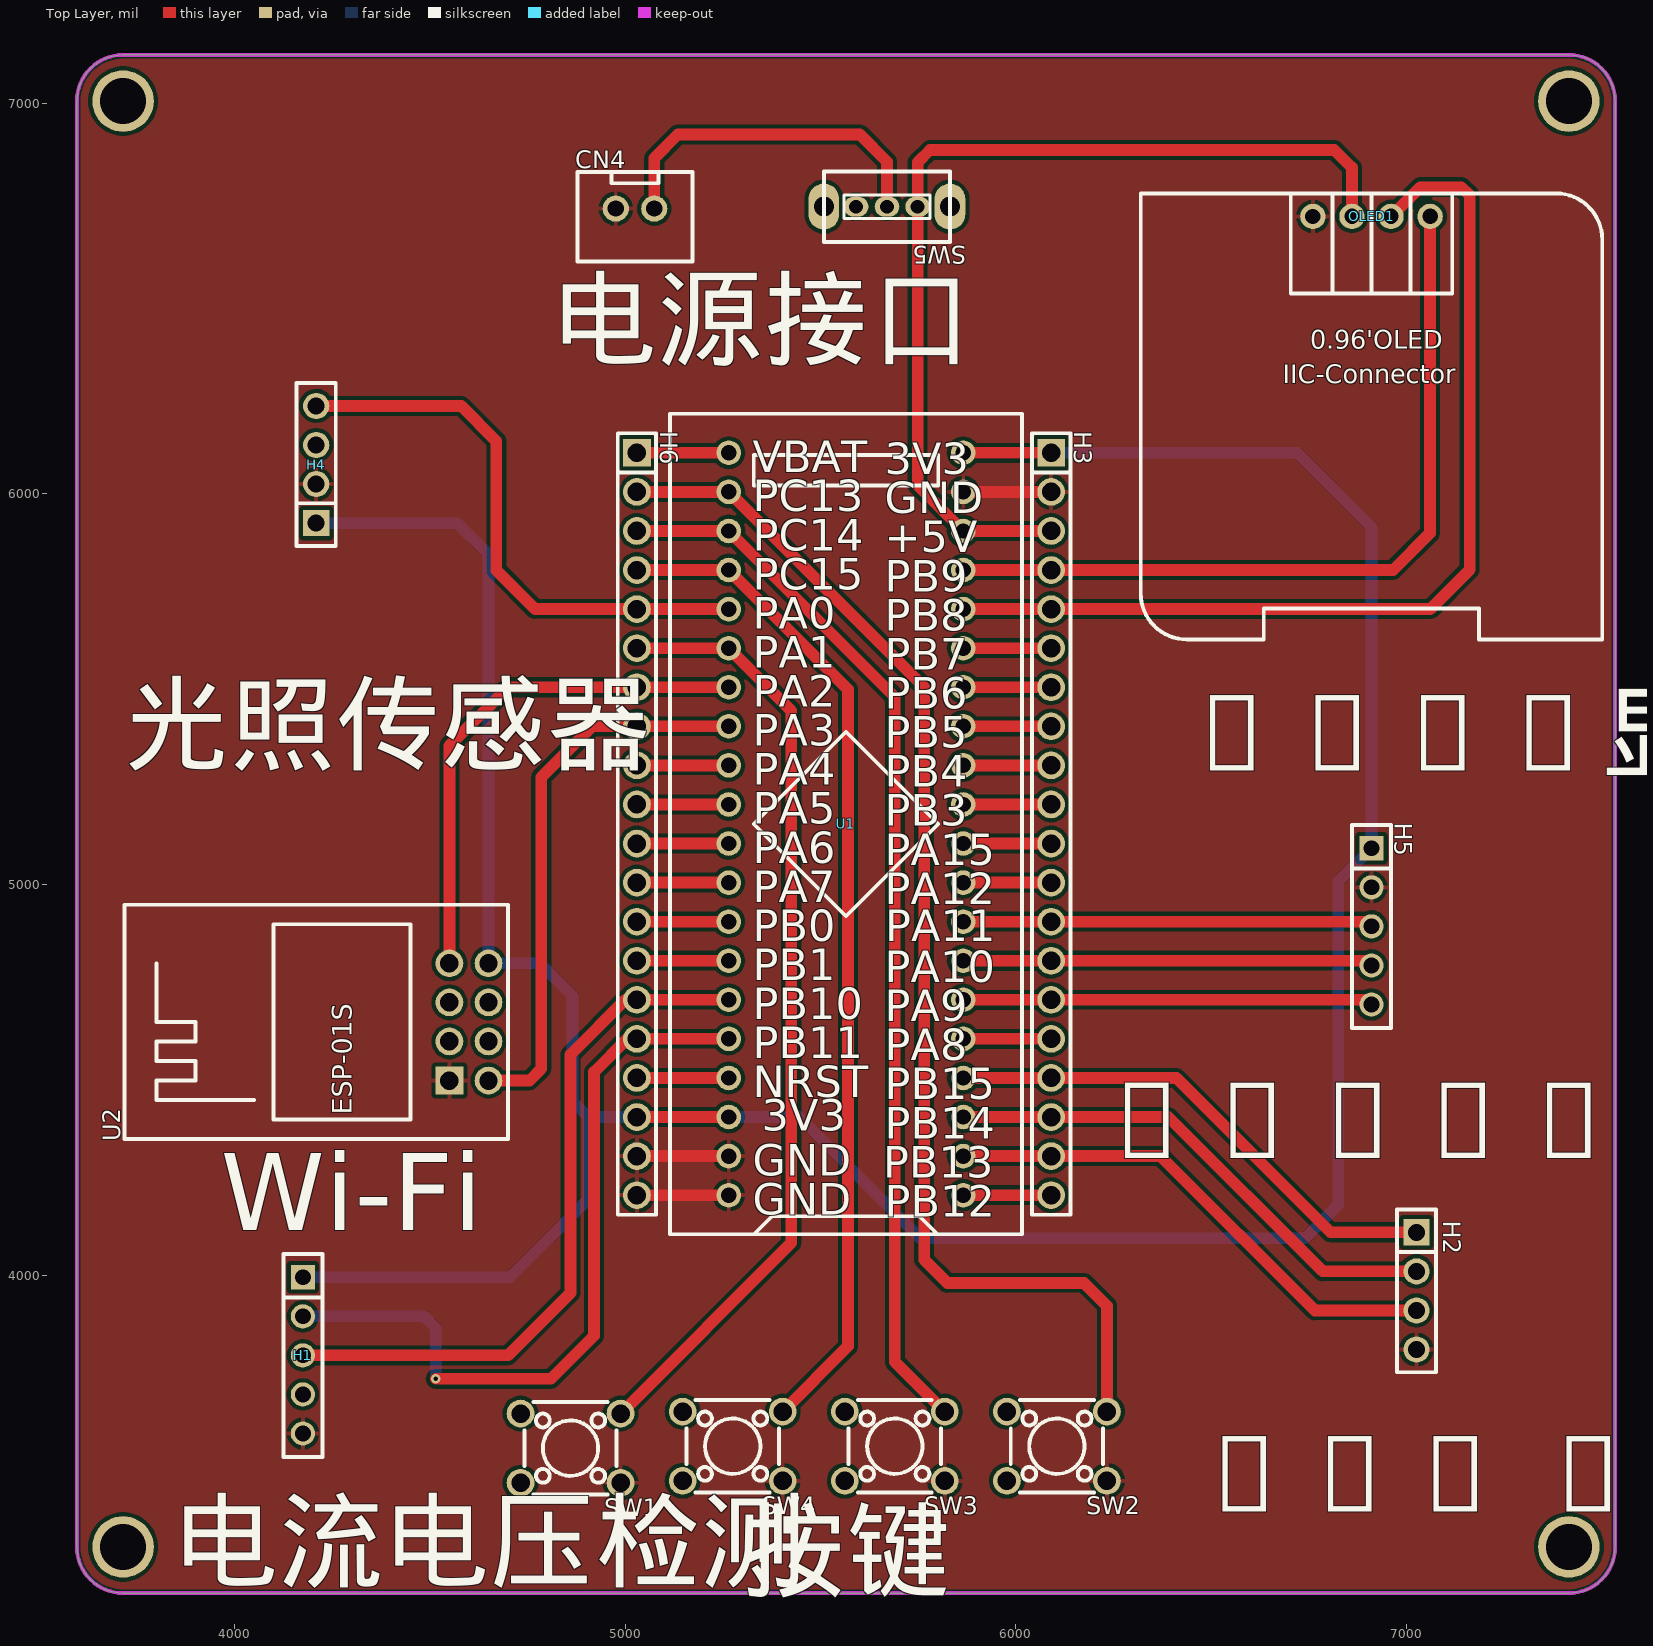
[diagram p0: Top Layer view]
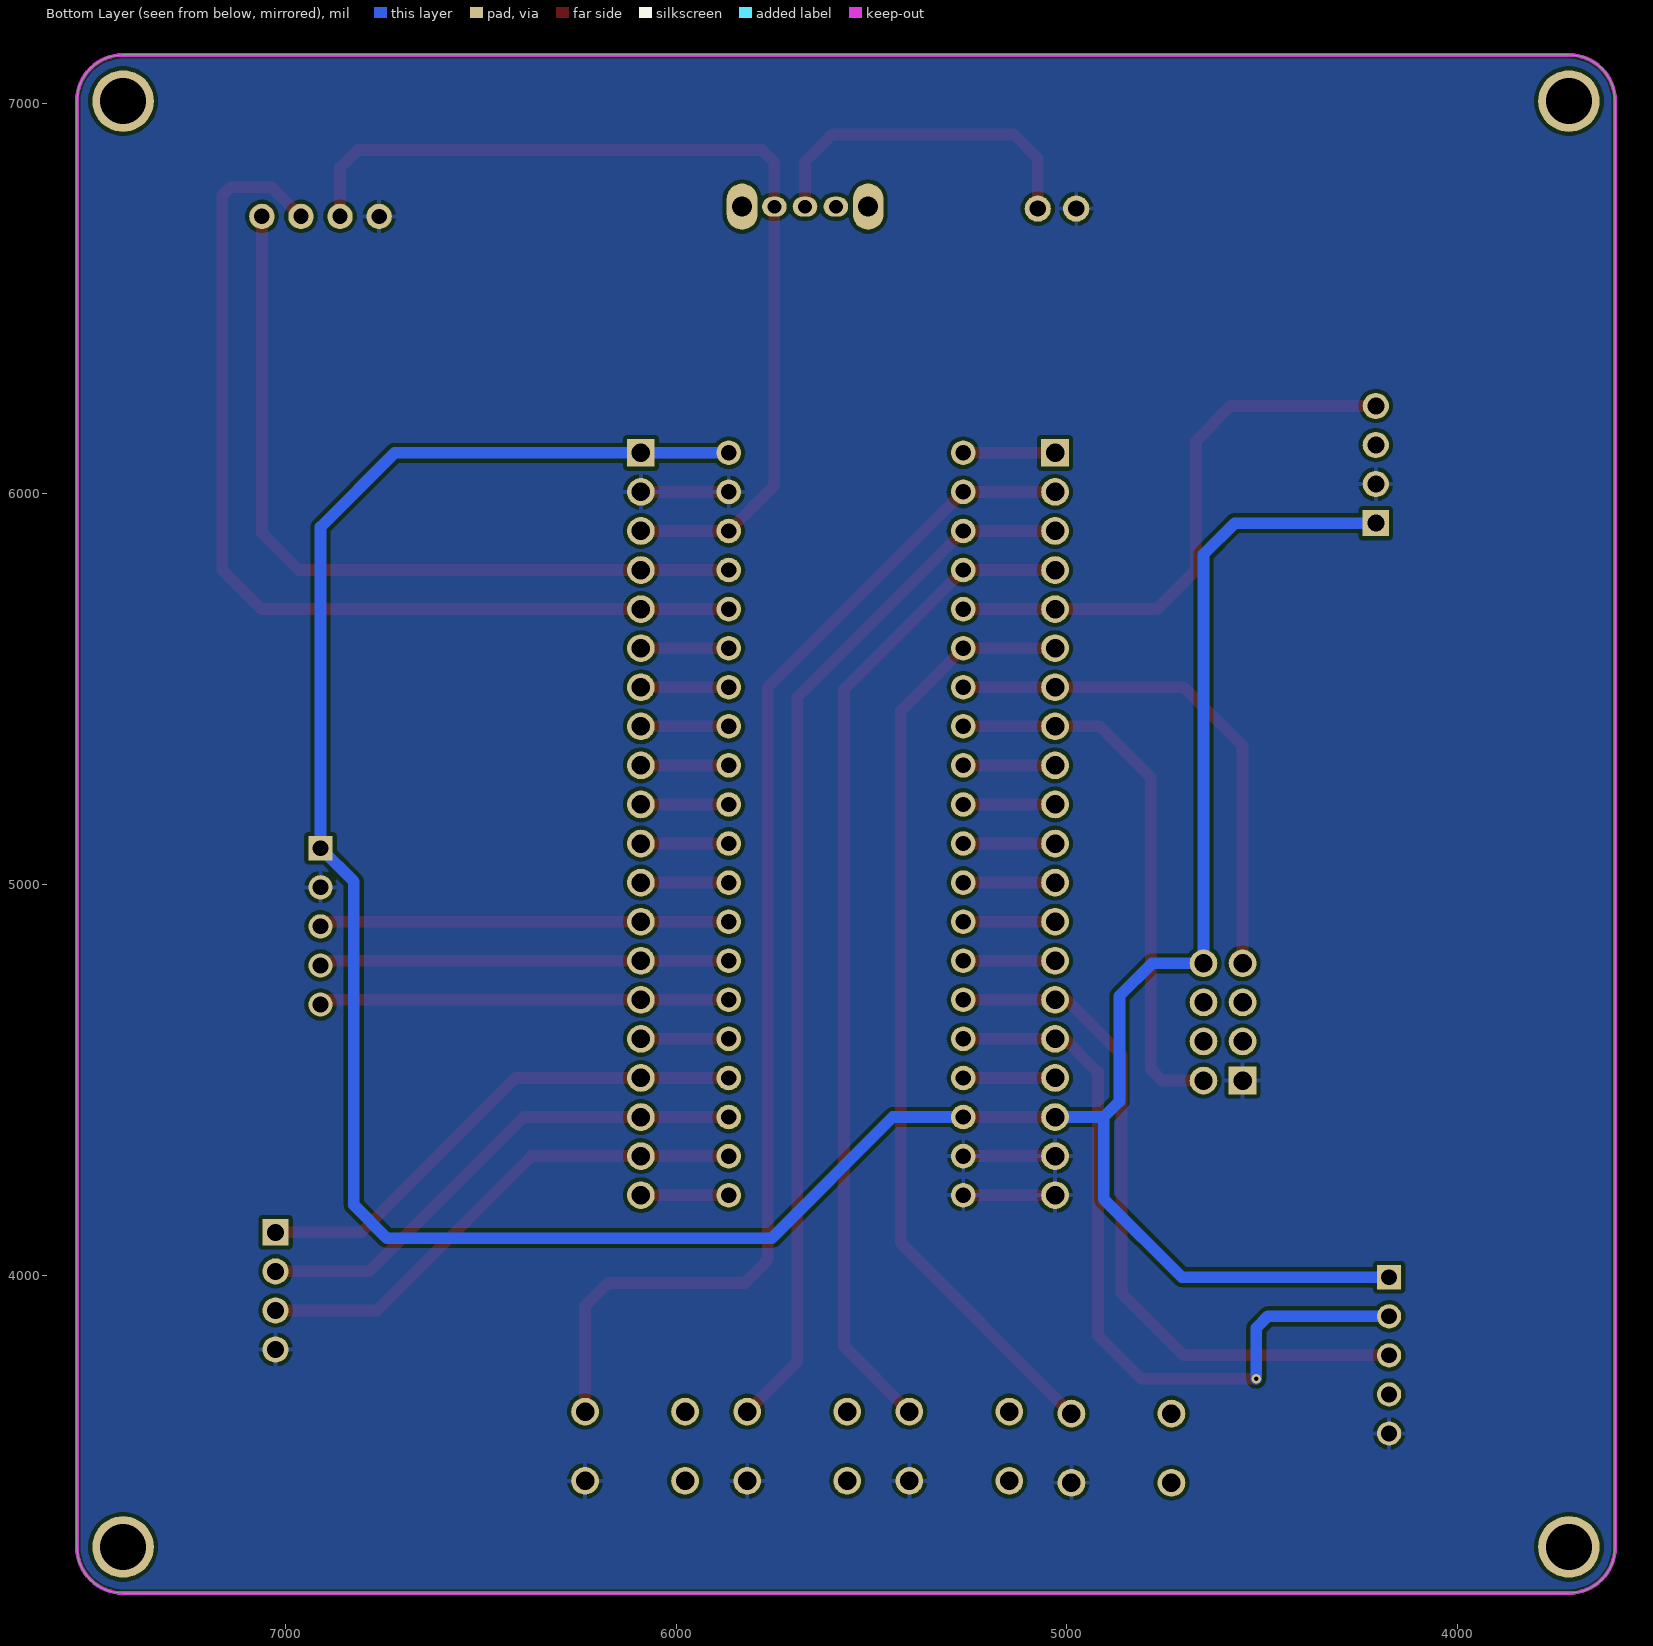
[diagram p1: Bottom Layer view, seen from below]
# Altium PCB MISC51840.pcbdoc
Units mil, origin at the board's own origin, x right, y up, seen from the top; angles counter-clockwise.
Board outline 3937.01 x 3937.01 mil, 2 copper layers (Top Layer, Bottom Layer), stack 62.206 mil thick; 15 components, 38 nets, 137 pads, 1 vias.

## Layer stack, top to bottom
Top Solder Mask Layer: solder mask 0.394, Dk 3.3
Top Layer: signal copper 1.379
Dielectric1: surface 59.449, FR4, Dk 4.5
Bottom Layer: signal copper 1.378
Bottom Solder Mask Layer: solder mask 0.394, Dk 3.3

## Board outline
3714.61,7123.5 ccw(c3714.61,7005.39) 3596.5,7005.39 3596.5,3304.61 ccw(c3714.61,3304.61) 3714.61,3186.5 7415.39,3186.5 ccw(c7415.39,3304.61) 7533.5,3304.61 7533.5,7005.39 ccw(c7415.39,7005.39) 7415.39,7123.5 3714.61,7123.5

## Design rules (kind name [scope] priority, off if disabled: settings)
BoardOutlineClearance copperThickness2oz_1 [All] p2 off: genericclearance=7.99 ignorepadtopadclearanceinfootprint=FALSE except(0: Arc-SplitContinuation Track-SplitContinuation SMDPad-SplitContinuation THPad-SplitContinuation Via-SplitContinuation Fill-SplitContinuation Region-SplitContinuation Poly-SplitContinuation Text-SplitContinuation Hole-SplitContinuation; 5.98: Arc-CutoutEdge Track-CutoutEdge SMDPad-CutoutEdge THPad-CutoutEdge Via-CutoutEdge Text-CutoutEdge; 6.9: Hole-OutlineEdge Hole-CutoutEdge; 10: Poly-OutlineEdge Poly-CutoutEdge; 11.81: Arc-OutlineEdge Track-OutlineEdge SMDPad-OutlineEdge THPad-OutlineEdge Via-OutlineEdge Fill-OutlineEdge Region-OutlineEdge Text-OutlineEdge Fill-CutoutEdge Region-CutoutEdge)
BoardOutlineClearance Plane_innerPlane_1 [All] p4 off: genericclearance=4.02 ignorepadtopadclearanceinfootprint=FALSE except(0: Arc-SplitContinuation Track-SplitContinuation SMDPad-SplitContinuation THPad-SplitContinuation Via-SplitContinuation Fill-SplitContinuation Region-SplitContinuation Poly-SplitContinuation Text-SplitContinuation Hole-SplitContinuation; 5.98: Arc-CutoutEdge Track-CutoutEdge SMDPad-CutoutEdge THPad-CutoutEdge Via-CutoutEdge Text-CutoutEdge; 6.9: Hole-OutlineEdge Hole-CutoutEdge; 10: Poly-OutlineEdge Poly-CutoutEdge; 11.81: Arc-OutlineEdge Track-OutlineEdge SMDPad-OutlineEdge THPad-OutlineEdge Via-OutlineEdge Fill-OutlineEdge Region-OutlineEdge Text-OutlineEdge Fill-CutoutEdge Region-CutoutEdge)
BoardOutlineClearance Copper_copperRegion_1 [All] p6 off: genericclearance=4.02 ignorepadtopadclearanceinfootprint=FALSE except(0: Arc-SplitContinuation Track-SplitContinuation SMDPad-SplitContinuation THPad-SplitContinuation Via-SplitContinuation Fill-SplitContinuation Region-SplitContinuation Poly-SplitContinuation Text-SplitContinuation Hole-SplitContinuation; 5.98: Arc-CutoutEdge Track-CutoutEdge SMDPad-CutoutEdge THPad-CutoutEdge Via-CutoutEdge Text-CutoutEdge; 6.9: Hole-OutlineEdge Hole-CutoutEdge; 10: Poly-OutlineEdge Poly-CutoutEdge; 11.81: Arc-OutlineEdge Track-OutlineEdge SMDPad-OutlineEdge THPad-OutlineEdge Via-OutlineEdge Fill-OutlineEdge Region-OutlineEdge Text-OutlineEdge Fill-CutoutEdge Region-CutoutEdge)
BoardOutlineClearance Copper_copperRegion_copperThickness1oz_1 [All] p8 off: genericclearance=4.02 ignorepadtopadclearanceinfootprint=FALSE except(0: Arc-SplitContinuation Track-SplitContinuation SMDPad-SplitContinuation THPad-SplitContinuation Via-SplitContinuation Fill-SplitContinuation Region-SplitContinuation Poly-SplitContinuation Text-SplitContinuation Hole-SplitContinuation; 5.98: Arc-CutoutEdge Track-CutoutEdge SMDPad-CutoutEdge THPad-CutoutEdge Via-CutoutEdge Text-CutoutEdge; 6.9: Hole-OutlineEdge Hole-CutoutEdge; 10: Poly-OutlineEdge Poly-CutoutEdge; 11.81: Arc-OutlineEdge Track-OutlineEdge SMDPad-OutlineEdge THPad-OutlineEdge Via-OutlineEdge Fill-OutlineEdge Region-OutlineEdge Text-OutlineEdge Fill-CutoutEdge Region-CutoutEdge)
BoardOutlineClearance Copper_copperRegion_Copper_copperRegion_1 [All] p10 off: genericclearance=4.02 ignorepadtopadclearanceinfootprint=FALSE except(0: Arc-SplitContinuation Track-SplitContinuation SMDPad-SplitContinuation THPad-SplitContinuation Via-SplitContinuation Fill-SplitContinuation Region-SplitContinuation Poly-SplitContinuation Text-SplitContinuation Hole-SplitContinuation; 5.98: Arc-CutoutEdge Track-CutoutEdge SMDPad-CutoutEdge THPad-CutoutEdge Via-CutoutEdge Text-CutoutEdge; 6.9: Hole-OutlineEdge Hole-CutoutEdge; 10: Poly-OutlineEdge Poly-CutoutEdge; 11.81: Arc-OutlineEdge Track-OutlineEdge SMDPad-OutlineEdge THPad-OutlineEdge Via-OutlineEdge Fill-OutlineEdge Region-OutlineEdge Text-OutlineEdge Fill-CutoutEdge Region-CutoutEdge)
BoardOutlineClearance copperThickness1oz_1 [All] p12: genericclearance=4.02 ignorepadtopadclearanceinfootprint=FALSE except(0: Arc-SplitContinuation Track-SplitContinuation SMDPad-SplitContinuation THPad-SplitContinuation Via-SplitContinuation Fill-SplitContinuation Region-SplitContinuation Poly-SplitContinuation Text-SplitContinuation Hole-SplitContinuation; 5.98: Arc-CutoutEdge Track-CutoutEdge SMDPad-CutoutEdge THPad-CutoutEdge Via-CutoutEdge Text-CutoutEdge; 6.9: Hole-OutlineEdge Hole-CutoutEdge; 10: Poly-OutlineEdge Poly-CutoutEdge; 11.81: Arc-OutlineEdge Track-OutlineEdge SMDPad-OutlineEdge THPad-OutlineEdge Via-OutlineEdge Fill-OutlineEdge Region-OutlineEdge Text-OutlineEdge Fill-CutoutEdge Region-CutoutEdge)
Clearance copperThickness2oz [All] p1 off: gap=7.99 ignorepadtopadclearanceinfootprint=FALSE except(5.98: SMDPad-Track SMDPad-SMDPad THPad-Track SMDPad-THPad THPad-THPad Track-Via SMDPad-Via THPad-Via Via-Via Fill-SMDPad Region-SMDPad Fill-THPad Region-THPad Fill-Via Region-Via Fill-Fill Fill-Region Region-Region Arc-Track Arc-SMDPad Arc-THPad Arc-Via Fill-Arc Region-Arc Arc-Arc Text-Track SMDPad-Text Text-THPad Text-Via Fill-Text Region-Text Arc-Text Text-Text; 6.9: Hole-Track Hole-SMDPad Hole-THPad Hole-Via Fill-Hole Region-Hole Hole-Arc Hole-Text; 10: Poly-Track Poly-SMDPad Poly-THPad Poly-Via Poly-Fill Poly-Region Poly-Poly Poly-Arc Poly-Text Poly-Hole; 11.81: Fill-Track Region-Track)
Clearance Plane_innerPlane [All] p3 off: gap=4.02 ignorepadtopadclearanceinfootprint=FALSE except(5.98: SMDPad-Track SMDPad-SMDPad THPad-Track SMDPad-THPad THPad-THPad Track-Via SMDPad-Via THPad-Via Via-Via Fill-SMDPad Region-SMDPad Fill-THPad Region-THPad Fill-Via Region-Via Fill-Fill Fill-Region Region-Region Arc-Track Arc-SMDPad Arc-THPad Arc-Via Fill-Arc Region-Arc Arc-Arc Text-Track SMDPad-Text Text-THPad Text-Via Fill-Text Region-Text Arc-Text Text-Text; 6.9: Hole-Track Hole-SMDPad Hole-THPad Hole-Via Fill-Hole Region-Hole Hole-Arc Hole-Text; 10: Poly-Track Poly-SMDPad Poly-THPad Poly-Via Poly-Fill Poly-Region Poly-Poly Poly-Arc Poly-Text Poly-Hole; 11.81: Fill-Track Region-Track)
Clearance Copper_copperRegion [All] p5 off: gap=4.02 ignorepadtopadclearanceinfootprint=FALSE except(5.98: SMDPad-Track SMDPad-SMDPad THPad-Track SMDPad-THPad THPad-THPad Track-Via SMDPad-Via THPad-Via Via-Via Fill-SMDPad Region-SMDPad Fill-THPad Region-THPad Fill-Via Region-Via Fill-Fill Fill-Region Region-Region Arc-Track Arc-SMDPad Arc-THPad Arc-Via Fill-Arc Region-Arc Arc-Arc Text-Track SMDPad-Text Text-THPad Text-Via Fill-Text Region-Text Arc-Text Text-Text; 6.9: Hole-Track Hole-SMDPad Hole-THPad Hole-Via Fill-Hole Region-Hole Hole-Arc Hole-Text; 10: Poly-Track Poly-SMDPad Poly-THPad Poly-Via Poly-Fill Poly-Region Poly-Poly Poly-Arc Poly-Text Poly-Hole; 11.81: Fill-Track Region-Track)
Clearance Copper_copperRegion_copperThickness1oz [All] p7 off: gap=4.02 ignorepadtopadclearanceinfootprint=FALSE except(5.98: SMDPad-Track SMDPad-SMDPad THPad-Track SMDPad-THPad THPad-THPad Track-Via SMDPad-Via THPad-Via Via-Via Fill-SMDPad Region-SMDPad Fill-THPad Region-THPad Fill-Via Region-Via Fill-Fill Fill-Region Region-Region Arc-Track Arc-SMDPad Arc-THPad Arc-Via Fill-Arc Region-Arc Arc-Arc Text-Track SMDPad-Text Text-THPad Text-Via Fill-Text Region-Text Arc-Text Text-Text; 6.9: Hole-Track Hole-SMDPad Hole-THPad Hole-Via Fill-Hole Region-Hole Hole-Arc Hole-Text; 10: Poly-Track Poly-SMDPad Poly-THPad Poly-Via Poly-Fill Poly-Region Poly-Poly Poly-Arc Poly-Text Poly-Hole; 11.81: Fill-Track Region-Track)
Clearance Copper_copperRegion_Copper_copperRegion [All] p9 off: gap=4.02 ignorepadtopadclearanceinfootprint=FALSE except(5.98: SMDPad-Track SMDPad-SMDPad THPad-Track SMDPad-THPad THPad-THPad Track-Via SMDPad-Via THPad-Via Via-Via Fill-SMDPad Region-SMDPad Fill-THPad Region-THPad Fill-Via Region-Via Fill-Fill Fill-Region Region-Region Arc-Track Arc-SMDPad Arc-THPad Arc-Via Fill-Arc Region-Arc Arc-Arc Text-Track SMDPad-Text Text-THPad Text-Via Fill-Text Region-Text Arc-Text Text-Text; 6.9: Hole-Track Hole-SMDPad Hole-THPad Hole-Via Fill-Hole Region-Hole Hole-Arc Hole-Text; 10: Poly-Track Poly-SMDPad Poly-THPad Poly-Via Poly-Fill Poly-Region Poly-Poly Poly-Arc Poly-Text Poly-Hole; 11.81: Fill-Track Region-Track)
Clearance copperThickness1oz [All] p11: gap=4.02 ignorepadtopadclearanceinfootprint=FALSE except(5.98: SMDPad-Track SMDPad-SMDPad THPad-Track SMDPad-THPad THPad-THPad Track-Via SMDPad-Via THPad-Via Via-Via Fill-SMDPad Region-SMDPad Fill-THPad Region-THPad Fill-Via Region-Via Fill-Fill Fill-Region Region-Region Arc-Track Arc-SMDPad Arc-THPad Arc-Via Fill-Arc Region-Arc Arc-Arc Text-Track SMDPad-Text Text-THPad Text-Via Fill-Text Region-Text Arc-Text Text-Text; 6.9: Hole-Track Hole-SMDPad Hole-THPad Hole-Via Fill-Hole Region-Hole Hole-Arc Hole-Text; 10: Poly-Track Poly-SMDPad Poly-THPad Poly-Via Poly-Fill Poly-Region Poly-Poly Poly-Arc Poly-Text Poly-Hole; 11.81: Fill-Track Region-Track)
DiffPairsRouting differentialPair [All] p1: maxlimit=6 minlimit=6 mostfreqgap=6 toplayer_minwidth=5 toplayer_prefwidth=10 toplayer_maxwidth=100 toplayer_mingap=6 toplayer_prefgap=6 toplayer_maxgap=6 bottomlayer_minwidth=5 bottomlayer_prefwidth=10 bottomlayer_maxwidth=100 bottomlayer_mingap=6 bottomlayer_prefgap=6 bottomlayer_maxgap=6 maxuncoupledlength=10
HoleToHoleClearance otherClearance [All] p1: gap=11.81 allowstackedmicrovias=TRUE
Length netLength [All] p1: minlimit=0 maxlimit=0
PasteMaskExpansion pasteMaskExpansion [All] p1: expansion=0
PlaneConnect innerPlane [All] p1: planeconnectstyle=Relief reliefexpansion=20 reliefentries=4 reliefconductorwidth=10 reliefairgap=10
PolygonConnect copperRegion_copperThickness1oz [All] p1 off: connectstyle=Relief reliefconductorwidth=10 reliefentries=4 polygonreliefangle="90 Angle" airgapwidth=10 via.connectstyle=Relief via.reliefconductorwidth=10 via.reliefentries=4 via.polygonreliefangle="90 Angle" via.airgapwidth=10
PolygonConnect copperRegion_Copper_copperRegion [All] p2 off: connectstyle=Relief reliefconductorwidth=10 reliefentries=4 polygonreliefangle="90 Angle" airgapwidth=10 via.connectstyle=Relief via.reliefconductorwidth=10 via.reliefentries=4 via.polygonreliefangle="90 Angle" via.airgapwidth=10
PolygonConnect copperRegion [All] p3: connectstyle=Relief reliefconductorwidth=10 reliefentries=4 polygonreliefangle="90 Angle" airgapwidth=10 via.connectstyle=Relief via.reliefconductorwidth=10 via.reliefentries=4 via.polygonreliefangle="90 Angle" via.airgapwidth=10
RoutingVias viaSize [All] p1: holewidth=12.01 width=24.02 viastyle="Through Hole" minholewidth=11.81 minwidth=19.68 maxholewidth=248.03 maxwidth=393.7
SolderMaskExpansion solderMaskExpansion [IsVia] p1: expansion=-1000 istentingtop=TRUE
SolderMaskExpansion solderMaskExpansion [All] p2: expansion=2 istentingtop=FALSE
Width copperThickness2oz_2 [All] p1 off: maxlimit=100 minlimit=8 preferedwidth=10
Width copperThickness1oz_2 [All] p2: maxlimit=100 minlimit=5 preferedwidth=10

## Components (designator, comment, footprint, x,y, rotation, side; value= is the part's Value field where it differs from the comment)
CN4 "XH2.54*2P_直插" CONN-TH_2P-P2.50-XH2.54-2P 5025,6730 r0 top
H1 "" HDR-TH_5P-P2.54-V-F 4175,3795 r270 top
H2 "" HDR-TH_4P-P2.54-V-F 7025,3960 r270 top
H3 "" HDR-TH_20P-P2.54-V-M-1 6090,5155 r270 top
H4 "" HDR-TH_4P-P2.54-V-F 4209,6075 r90 top
H5 "" HDR-TH_5P-P2.54-V-F 6910,4892.92 r270 top
H6 "" HDR-TH_20P-P2.54-V-M-1 5030,5155 r270 top
OLED1 "" 0.96OLED_4P 6910,6710 r0 top
SW1 "" SW-TH_4P-L6.0-W6.0-P4.50-LS6.5 4860,3557.47 r180 top
SW2 "" SW-TH_4P-L6.0-W6.0-P4.50-LS6.5 6104.85,3562.47 r180 top
SW3 "" SW-TH_4P-L6.0-W6.0-P4.50-LS6.5 5689.9,3562.47 r180 top
SW4 "" SW-TH_4P-L6.0-W6.0-P4.50-LS6.5 5274.95,3562.47 r180 top
SW5 "" 拨动开关 5675,6735 r180 top
U1 "STM32F103C8T6-Card" CONN-TH_L53.3-W22.9_STM32F103C8T6-CARD 5565,5155 r90 top
U2 "ESP-01S" WIFIM-TH_ESP-01S 4600,4648.39 r90 top

## Footprints (in the part's own frame and the unit in brackets; to place one, negate y for a bottom-side part, rotate by r counter-clockwise, add the part's x,y. Pads: shape width x height; smd on the part's side, far side on the other; paste and mask are expansions set on the pad)
0.96OLED_4P [mm]
  round 1.65 hole 1 copper offset 0,0: 1(-3.81,-0.001) 2(-1.27,0.002) 3(1.27,0.002) 4(3.81,0.002)
  silkscreen extent -15,-27.5 15,1.5
CONN-TH_2P-P2.50-XH2.54-2P [mm]
  round 1.7 hole 1.05 paste+0 mask+0.05: 1(1.25,0) 2(-1.25,0)
  silkscreen extent -3.75,-3.42 3.75,2.37
CONN-TH_L53.3-W22.9_STM32F103C8T6-CARD [mm]
  round 1.6 hole 1: 1(-24.13,-7.62) 2(-21.59,-7.62) 3(-19.05,-7.62) 4(-16.51,-7.62) 5(-13.97,-7.62) 6(-11.43,-7.62) 7(-8.89,-7.62) 8(-6.35,-7.62) 9(-3.81,-7.62) 10(-1.27,-7.62) 11(1.27,-7.62) 12(3.81,-7.62) 13(6.35,-7.62) 14(8.89,-7.62) 15(11.43,-7.62) 16(13.97,-7.62) 17(16.51,-7.62) 18(19.05,-7.62) 19(21.59,-7.62) 20(24.13,-7.62) 21(24.13,7.62) 22(21.59,7.62) 23(19.05,7.62) 24(16.51,7.62) 25(13.97,7.62) 26(11.43,7.62) 27(8.89,7.62) 28(6.35,7.62) 29(3.81,7.62) 30(1.27,7.62) 31(-1.27,7.62) 32(-3.81,7.62) 33(-6.35,7.62) 34(-8.89,7.62) 35(-11.43,7.62) 36(-13.97,7.62) 37(-16.51,7.62) 38(-19.05,7.62) 39(-21.59,7.62) 40(-24.13,7.62)
  silkscreen extent -26.67,-11.43 26.67,11.43
HDR-TH_4P-P2.54-V-F [mm]
  rect 1.7x1.7 hole 1.1: 1(-3.81,0)
  round 1.7 hole 1.1: 2(-1.27,0) 3(1.27,0) 4(3.81,0)
  silkscreen extent -5.29,-1.27 5.29,1.27
HDR-TH_5P-P2.54-V-F [mil]
  rect 62x62 hole 40.16: 1(-200,0)
  round 62 hole 40.16: 2(-100,0) 3(0,0) 4(100,0) 5(200,0)
  silkscreen extent -260,-50 260,50
HDR-TH_20P-P2.54-V-M-1 [mm]
  rect 1.8x1.8 hole 1.2: 1(-24.13,0)
  round 1.8 hole 1.2: 2(-21.59,0) 3(-19.05,0) 4(-16.51,0) 5(-13.97,0) 6(-11.43,0) 7(-8.89,0) 8(-6.35,0) 9(-3.81,0) 10(-1.27,0) 11(1.27,0) 12(3.81,0) 13(6.35,0) 14(8.89,0) 15(11.43,0) 16(13.97,0) 17(16.51,0) 18(19.05,0) 19(21.59,0) 20(24.13,0)
  silkscreen extent -25.4,-1.25 25.4,1.25
SW-TH_4P-L6.0-W6.0-P4.50-LS6.5 [mm]
  round 1.8 hole 1.2: 1(-3.25,2.25) 2(3.25,2.25) 3(-3.25,-2.25) 4(3.25,-2.25)
  silkscreen extent -3,-3 3,3
WIFIM-TH_ESP-01S [mm]
  rect 1.8x1.8 hole 1.2: 1(-3.81,1.27)
  round 1.8 hole 1.2: 2(-1.27,1.27) 3(1.27,1.27) 4(3.81,1.27) 5(3.81,-1.27) 6(1.27,-1.27) 7(-1.27,-1.27) 8(-3.81,-1.27)
  silkscreen extent -7.62,-2.54 7.62,22.4
拨动开关 [mil]
  oval 63x51.2 hole 35.4 paste+0 mask+2: 1(-73.4,0) 2(5,0) 3(84,0)
  oval 78.7x118.1 hole 51.2 paste+0 mask+2: 4(166.7,0) 5(-156.1,0)
  silkscreen extent -156,-90 167,90

## Free pads (board coordinates)
  round 157.48 hole 118.11: 1(3714.61,7005.39) 1(3714.61,3304.61) 1(7415.39,7005.39) 1(7415.39,3304.61)

## Via types
v1: diameter 24.02, hole 12, Top Layer to Bottom Layer, 1 vias

## Nets (pads, with @x,y where several pads share a name; then routed paths per layer and width w, separated by ;. In a path a pad name is that pad's centre, name@x,y a point inside that pad or via, vN(x,y) a via of type N, cw(c..) or ccw(c..) an arc to the next point about the centre after c; other vN are vias at no path point)
$1N17153: CN4.1 SW5.2 | length 894.2
  Top Layer w30: CN4.1 5074.22,6859.22 5135,6920 5600,6920 5670,6850 SW5.2
+5V: H3.3 OLED1.2 SW5.1 U1.18 | length 2495
  Top Layer w30: H3.3@6100,5905 U1.18 5748.4,6021.6 SW5.1 5748.4,6848.4 5780,6880 6815,6880 6860,6835 OLED1.2@6860,6710.05
GND: CN4.2 H1.5 H2.4 H3.2 H4.2 H5.2 H6.19 H6.20 OLED1.1 SW1.1 SW2.1 SW3.1 SW4.1 U1.19 U1.39 U1.40 U2.1 | length 725
  Top Layer w30: H6.20@5020,4205 U1.40 ; H6.19@5020,4305 U1.39 ; U1.19 H3.2@6100,6005
NRST: H6.17 U1.37 | length 245
  Top Layer w30: H6.17@5020,4505 U1.37
PA0: H4.4 H6.5 U1.25 | length 1464.7
  Top Layer w30: H4.4 4580,6225 4670,6135 4670,5805 4770,5705 H6.5 U1.25
PA1: H6.6 SW1.3 U1.26 | length 2451.3
  Top Layer w30: SW1.3 5425,4083.1 5425,5445 U1.26 H6.6@5020,5605
PA2: H6.7 U1.27 U2.4 | length 1333.7
  Top Layer w30: U2.4 4550,5355 4700,5505 H6.7 U1.27
PA3: H6.8 U1.28 U2.8 | length 1427.9
  Top Layer w30: U2.8 4755,4498.39 4785,4528.39 4785,5275 4915,5405 H6.8 U1.28
PA4: H6.9 U1.29 | length 245
  Top Layer w30: H6.9@5020,5305 U1.29
PA5: H6.10 U1.30 | length 245
  Top Layer w30: H6.10@5020,5205 U1.30
PA6: H6.11 U1.31 | length 245
  Top Layer w30: H6.11@5020,5105 U1.31
PA7: H6.12 U1.32 | length 245
  Top Layer w30: H6.12@5020,5005 U1.32
PA8: H3.16 U1.5 | length 235
  Top Layer w30: U1.5 H3.16@6100,4605
PA9: H3.15 H5.5 U1.6 | length 1050
  Top Layer w30: U1.6 H3.15 6897.91,4705 H5.5
PA10: H3.14 H5.4 U1.7 | length 1050
  Top Layer w30: U1.7 H3.14 6897.91,4805 H5.4
PA11: H3.13 H5.3 U1.8 | length 1050
  Top Layer w30: U1.8 H3.13 6897.91,4905 H5.3
PA12: H3.12 U1.9 | length 235
  Top Layer w30: U1.9 H3.12@6100,5005
PA15: H3.11 U1.10 | length 235
  Top Layer w30: U1.10 H3.11@6100,5105
PB0: H6.13 U1.33 | length 245
  Top Layer w30: H6.13@5020,4905 U1.33
PB1: H6.14 U1.34 | length 245
  Top Layer w30: H6.14@5020,4805 U1.34
PB3: H3.10 U1.11 | length 235
  Top Layer w30: U1.11 H3.10@6100,5205
PB4: H3.9 U1.12 | length 235
  Top Layer w30: U1.12 H3.9@6100,5305
PB5: H3.8 U1.13 | length 235
  Top Layer w30: U1.13 H3.8@6100,5405
PB6: H3.7 U1.14 | length 235
  Top Layer w30: U1.14 H3.7@6100,5505
PB7: H3.6 U1.15 | length 235
  Top Layer w30: U1.15 H3.6@6100,5605
PB8: H3.5 OLED1.3 U1.16 | length 2536.8
  Top Layer w30: U1.16 H3.5 7060,5705 7161.21,5806.21 7161.21,6763.79 7140,6785 7034.95,6785 OLED1.3@6960,6710.05
PB9: H3.4 OLED1.4 U1.17 | length 2044.4
  Top Layer w30: U1.17 H3.4 6965,5805 7060,5900 OLED1.4@7060,6710.05
PB10: H1.3 H6.15 U1.35 | length 1824.3
  Top Layer w30: H1.3 4700,3795 4860,3955 4860,4565 5000,4705 U1.35
PB11: H1.2 H6.16 U1.36 | length 1988.2
  Top Layer w30: v1(4515,3735) 4810,3735 4920,3845 4920,4520 5005,4605 U1.36
  Bottom Layer w30: H1.2 4485,3895 4515,3865 v1(4515,3735)
PB12: H3.20 U1.1 | length 235
  Top Layer w30: U1.1 H3.20@6100,4205
PB13: H2.3 H3.19 U1.2 | length 1323.6
  Top Layer w30: U1.2 H3.19 6370,4305 6765,3910 H2.3
PB14: H2.2 H3.18 U1.3 | length 1323.6
  Top Layer w30: U1.3 H3.18 6390,4405 6785,4010 H2.2
PB15: H2.1 H3.17 U1.4 | length 1323.6
  Top Layer w30: U1.4 H3.17 6410,4505 6805,4110 H2.1
PC13: H6.2 SW2.3 U1.22 | length 3204.9
  Top Layer w30: H6.2@5020,6005 U1.22 5765,5505 5765,4040 5825,3980 6175,3980 6232.8,3922.2 SW2.3
PC14: H6.3 SW3.3 U1.23 | length 2727.9
  Top Layer w30: H6.3@5020,5905 U1.23 5690,5480 5690,3778.9 SW3.3@5817.85,3651.05
PC15: H6.4 SW4.3 U1.24 | length 2594.5
  Top Layer w30: H6.4@5020,5805 U1.24 5570,5500 5570,3818.15 SW4.3
VBAT: H6.1 U1.21 | length 245
  Top Layer w30: H6.1@5020,6105 U1.21
VCC: H1.1 H3.1 H4.1 H5.1 H6.18 U1.20 U1.38 U2.5 | length 8342.2
  Top Layer w30: H6.18@5020,4405 U1.38 ; U1.20 H3.1@6100,6105
  Bottom Layer w30: H1.1 4705,3995 4905,4195 4905,4405 ; H4.1 4570,5925 4650,5845 U2.5 4781.61,4798.39 4865,4715 4865,4445 4905,4405 ; H6.18 4905,4405 ; U1.38 5445,4405 5755,4095 6740,4095 6825,4180 6825,5007.92 H5.1 6910,5915 6720,6105 H3.1 U1.20
pads on no net: H1.4 H4.3 SW1.2 SW1.4 SW2.2 SW2.4 SW3.2 SW3.4 SW4.2 SW4.4 SW5.3 SW5.4 SW5.5 U2.2 U2.3 U2.6 U2.7

## Polygon pours and split planes (outlines as drawn)
GND on Bottom Layer (solid, remove dead copper, pour order 2): 3525,7245 3525,3080 7700,3080 7700,7245
GND on Top Layer (solid, remove dead copper, pour order 2): 3000,7415 3000,3000 7930,3000 7930,7415

## Keep-outs
Board Outline Layer:
  the board outline again, w10

## Silkscreen, mask and mechanical layers (free items; w line width, h text height)
Top Silkscreen Layer:
  text "电源接口" at 4812.87,6351.57 h196.85
  text "VBAT" at 5325.95,6055 h80
  text "3V3" at 5664.16,6050 h80
  text "PC13" at 5325.95,5955 h80
  text "GND" at 5664.16,5950 h80
  text "PC14" at 5325.95,5855 h80
  text "+5V" at 5664.16,5850 h80
  text "PC15" at 5325.95,5755 h80
  text "PB9" at 5664.16,5750 h80
  text "PA0" at 5325.95,5655 h80
  text "PB8" at 5664.16,5650 h80
  text "PA1" at 5325.95,5555 h80
  text "PB7" at 5664.16,5550 h80
  text "PA2" at 5325.95,5455 h80
  text "PB6" at 5664.16,5450 h80
  text "PA3" at 5325.95,5355 h80
  text "PB5" at 5664.16,5350 h80
  text "光照传感器" at 3718.07,5315 h196.85
  text "Oled显示器" at 6418.02,5291.63 h196.85
  text "PA4" at 5325.95,5255 h80
  text "PB4" at 5664.16,5250 h80
  text "PA5" at 5325.95,5155 h80
  text "PB3" at 5664.16,5150 h80
  text "PA6" at 5325.95,5055 h80
  text "PA15" at 5664.16,5050 h80
  text "PA7" at 5325.95,4955 h80
  text "PA12" at 5664.16,4950 h80
  text "PB0" at 5325.95,4855 h80
  text "PA11" at 5665.95,4855 h80
  text "PB1" at 5325.95,4755 h80
  text "PA10" at 5664.16,4750 h80
  text "PB10" at 5325.95,4655 h80
  text "PA9" at 5664.16,4650 h80
  text "PB11" at 5325.95,4555 h80
  text "PA8" at 5664.16,4550 h80
  text "NRST" at 5325.95,4455 h80
  text "PB15" at 5664.16,4450 h80
  text "3V3" at 5350,4370 h80
  text "PB14" at 5664.16,4350 h80
  text "DS1302实时时钟" at 6200,4300 h196.85
  text "GND" at 5325.95,4255 h80
  text "PB13" at 5660.95,4250 h80
  text "GND" at 5325.95,4155 h80
  text "PB12" at 5664.16,4150 h80
  text "Wi-Fi" at 3965,4115 h196.85
  text "RGB LED灯" at 6450,3395 h196.85
  text "电流电压检测" at 3845,3225 h196.85
  text "按键" at 5295,3200 h196.85